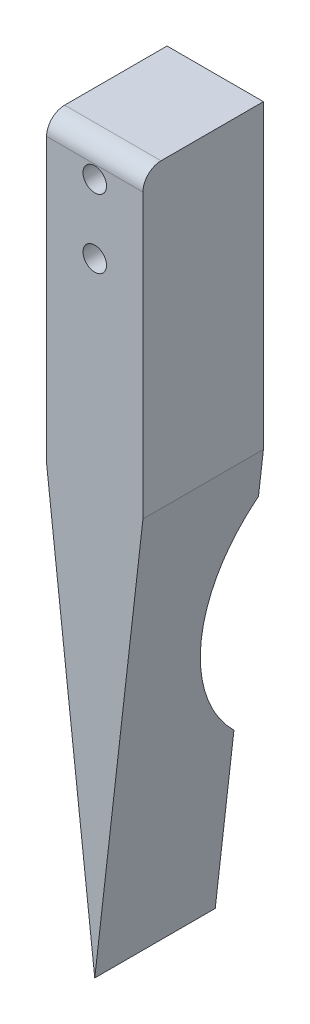
SolidWorks part; units mm, degrees
material "硅橡胶"
ref_plane "前视基准面" through (0, 0, 0) normal (0, 0, 1) x (1, 0, 0)
ref_plane "上视基准面" through (0, 0, 0) normal (0, 1, 0) x (1, 0, 0)
ref_plane "右视基准面" through (0, 0, 0) normal (1, 0, 0) x (0, 0, -1)
sketch "草图1" plane through (0, 0, 0) normal (0, 0, 1) x (1, 0, 0)
  line L0 (-4, 0) -> (4, 0)
  line L1 (-4, 0) -> (-4, -25)
  line L5 (4, -25) -> (4, 0)
  line L6 (0, -15) -> (0, -60) construction
  line L7 (-4, -25) -> (0, -60)
  line L8 (4, -25) -> (0, -60)
  point P4 (0, 0)
  dimension "D1" = 25
  dimension "D2" = 8
  dimension "D3" = 60
  dimension "D4" = 25
extrude "凸台-拉伸1" add sketch "草图1" along normal blind 10
sketch "草图3" plane through (0, 0, 10) normal (0, 0, 1) x (1, 0, 0)
  circle A0 centre (0, -8.2843) radius 0.975
  circle A1 centre (0, -2.5843) radius 0.975
extrude "切除-拉伸2" cut sketch "草图3" against normal through all
fillet "圆角1" radius 1.5 1 edges at (0, 0, 10)
sketch "草图6" plane through (-4, 0, 0) normal (-1, 0, 0) x (0, 0, 1)
  line L0 (10, -25) -> (0, -25) construction
  line L2 (0, -25) -> (0, -60) construction
  circle A0 centre (-8.77, -37.5) radius 12.5
  dimension "D1" = 25
  dimension "D2" = 12.5
  dimension "D3" = 8.77
extrude "切除-拉伸3" cut sketch "草图6" against normal through all both and the other way through all
